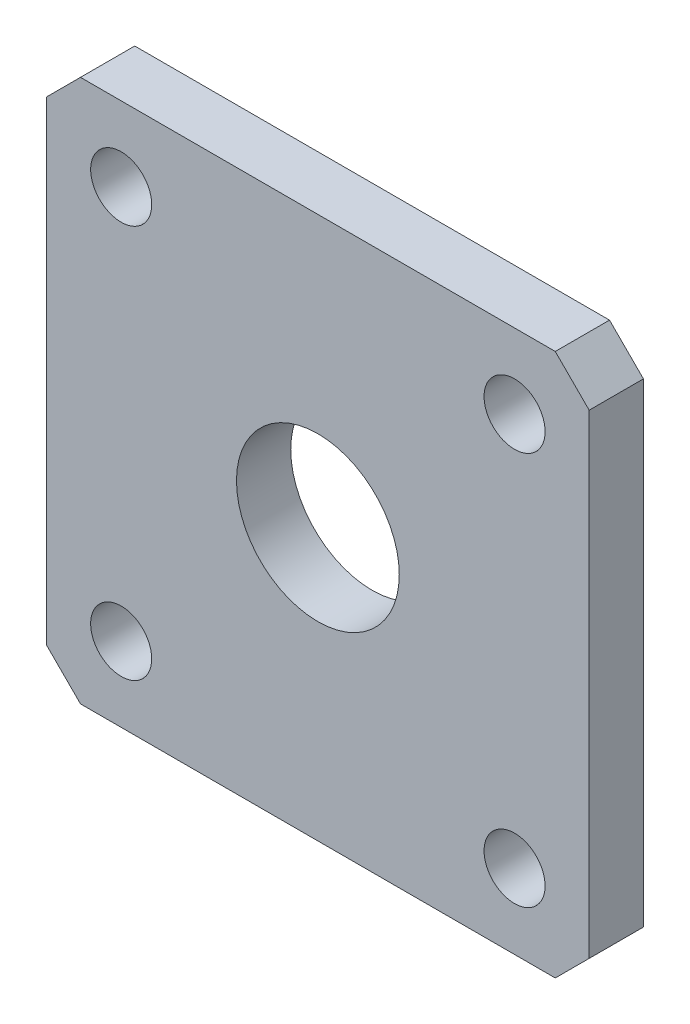
from build123d import *

# Parameters (mm, degrees)
SKETCH1_W           = 80
SKETCH1_H           = 80
SKETCH1_R           = 12
SKETCH1_R_2         = 4.5
BOSS_EXTRUDE1_DEPTH = 8
CHAMFER1_SIZE       = 5


with BuildPart() as part:
    # Sketch1 → Boss-Extrude1 (new body)
    with BuildSketch(Plane.XY):
        with Locations((-1.114398958, 9.473684211)):
            Rectangle(SKETCH1_W, SKETCH1_H)
        with Locations((-1.114398958, 9.473684211)):
            Circle(SKETCH1_R, mode=Mode.SUBTRACT)
        with Locations((-30.114398958, 38.473684211)):
            Circle(SKETCH1_R_2, mode=Mode.SUBTRACT)
        with Locations((-30.114398958, -19.526315789)):
            Circle(SKETCH1_R_2, mode=Mode.SUBTRACT)
        with Locations((27.885601042, -19.526315789)):
            Circle(SKETCH1_R_2, mode=Mode.SUBTRACT)
        with Locations((27.885601042, 38.473684211)):
            Circle(SKETCH1_R_2, mode=Mode.SUBTRACT)
    extrude(amount=BOSS_EXTRUDE1_DEPTH)

    # Chamfer1
    chamfer1_edges = [part.edges().sort_by_distance(p)[0] for p in [
        (-41.114398958, 49.473684211, 4),
        (38.885601042, 49.473684211, 4),
        (38.885601042, -30.526315789, 4),
        (-41.114398958, -30.526315789, 4),
    ]]
    chamfer(chamfer1_edges, length=CHAMFER1_SIZE)


solid = part.part
